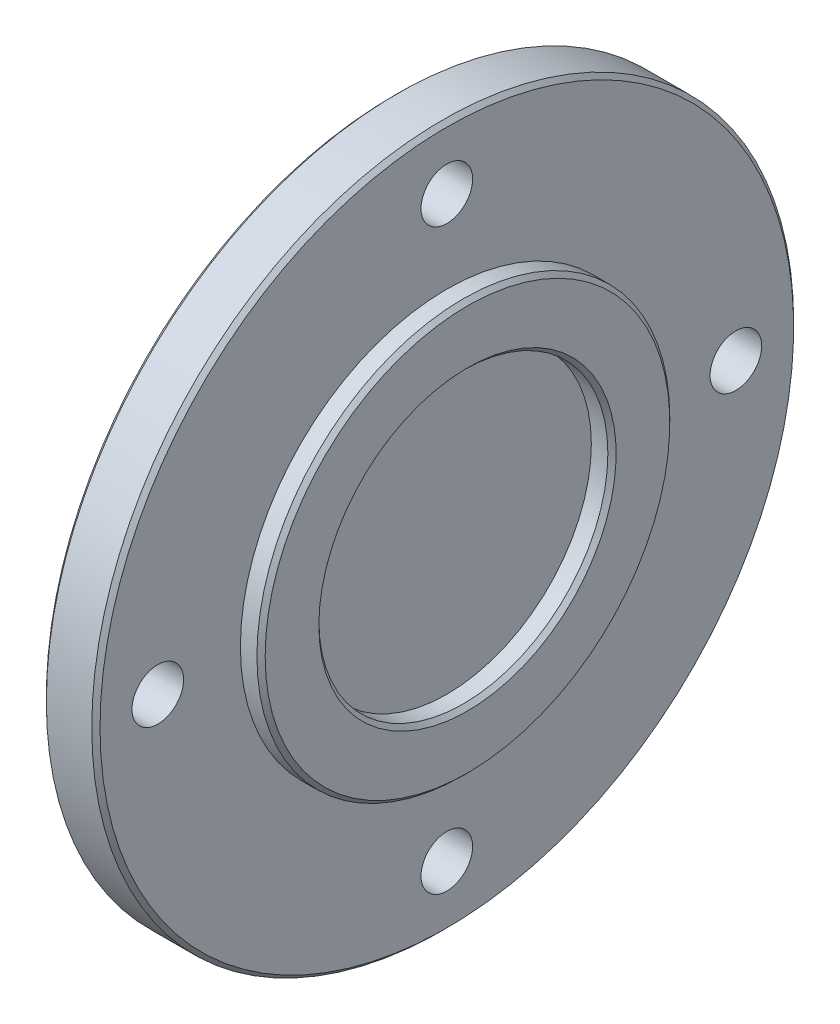
SolidWorks part; units mm, degrees
material "普通碳钢"
ref_plane "前视基准面" through (0, 0, 0) normal (0, 0, 1) x (1, 0, 0)
ref_plane "上视基准面" through (0, 0, 0) normal (0, 1, 0) x (1, 0, 0)
ref_plane "右视基准面" through (0, 0, 0) normal (1, 0, 0) x (0, 0, -1)
sketch "草图1" plane through (0, 0, 0) normal (0, 0, 1) x (1, 0, 0)
  line L0 (0, 0) -> (0, 290.7532) construction
  line L1 (0, 0) -> (356.4696, 0) construction
  line L2 (0, 0) -> (0, 85)
  line L3 (0, 85) -> (13, 85)
  line L4 (13, 85) -> (13, 50)
  line L5 (13, 50) -> (18, 50)
  line L6 (18, 50) -> (18, 35)
  line L7 (18, 35) -> (13, 35)
  line L8 (13, 35) -> (13, 0)
  line L9 (13, 0) -> (0, 0)
  dimension "D1" = 170
  dimension "D2" = 100
  dimension "D3" = 15
  dimension "D4" = 13
  dimension "D5" = 5
revolve "旋转1" add sketch "草图1" angle 360 about L1
sketch "草图2" plane through (0, 0, 0) normal (-1, 0, 0) x (0, 0, 1)
  line L0 (0, 0) -> (0, 70) construction
  circle A0 centre (0, 70) radius 6.25
  dimension "D2" = 12.5
  dimension "D1" = 70
extrude "切除-拉伸1" cut sketch "草图2" against normal through all
pattern_circular "阵列(圆周)1" count 4 over 360 about axis through (0, 0, 0) along (1, 0, 0) of "切除-拉伸1"
chamfer "倒角1" distance 1 angle 45 4 edges at (18, 0, 35) (18, 0, 50) (0, 0, 85) (13, 0, 85)
